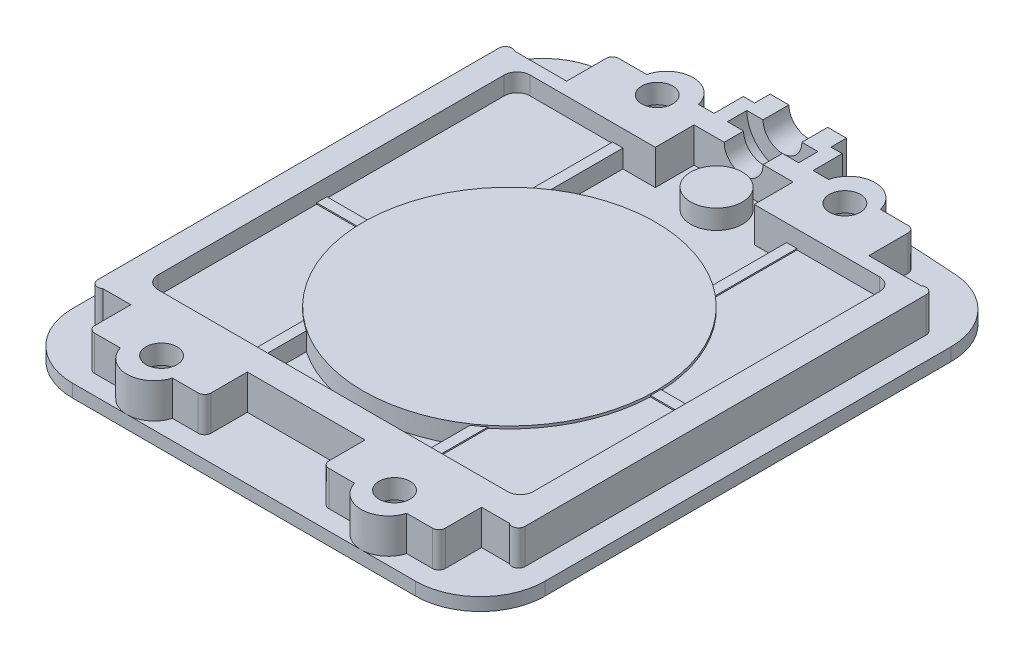
from build123d import *

# Parameters (mm, degrees)
BOSS_EXTRUDE1_DEPTH      = 1
BOSS_EXTRUDE3_DEPTH      = 2.7
BOSS_EXTRUDE3_DEPTH_BACK = 1
BOSS_EXTRUDE4_DEPTH      = 1.3
BOSS_EXTRUDE5_DEPTH      = 0.1
SKETCH_6_R               = 11.3
BOSS_EXTRUDE6_DEPTH      = 1.5
SKETCH_8_R               = 1.2
CUT_EXTRUDE1_DEPTH       = 3.7
SKETCH_9_R               = 1.85
SKETCH_9_R_2             = 9.175
CUT_EXTRUDE2_DEPTH       = 2.2
SKETCH_10_R              = 2
BOSS_EXTRUDE11_DEPTH     = 1.5


with BuildPart() as part:
    # Sketch 1 → Boss-Extrude1 (new body)
    with BuildSketch(Plane(origin=(0, 0, 0), x_dir=(1, 0, 0), z_dir=(0, 1, 0))):
        with BuildLine():
            Line((-13.25, -20.5), (13.25, -20.5))
            ThreePointArc((13.25, -20.5), (16.785533906, -19.035533906), (18.25, -15.5))
            Line((18.25, -15.5), (18.25, 15.890687558))
            ThreePointArc((18.25, 15.890687558), (16.905897578, 19.301613077), (13.59623484, 20.878685296))
            ThreePointArc((13.59623484, 20.878685296), (0, 21.35), (-13.59623484, 20.878685296))
            ThreePointArc((-13.59623484, 20.878685296), (-16.905897578, 19.301613077), (-18.25, 15.890687558))
            Line((-18.25, 15.890687558), (-18.25, -15.5))
            ThreePointArc((-18.25, -15.5), (-16.785533906, -19.035533906), (-13.25, -20.5))
        make_face()
    extrude(amount=BOSS_EXTRUDE1_DEPTH)

    # Sketch 2 → Boss-Extrude3 (add, two sides: drawn at the far end of the back side and taken through both)
    with BuildSketch(Plane(origin=(0, 1, 0), x_dir=(1, 0, 0), z_dir=(0, 1, 0)).offset(-BOSS_EXTRUDE3_DEPTH_BACK)):
        with BuildLine():
            Line((-13.55, -15.702154728), (-15.705804316, -15.702154728))
            ThreePointArc((-15.705804316, -15.702154728), (-16.229411113, -15.749368323), (-16.505804316, -15.302154728))
            Line((-16.505804316, -15.302154728), (-16.505804316, 15.697845272))
            ThreePointArc((-16.505804316, 15.697845272), (-16.229411113, 16.145058868), (-15.705804316, 16.097845272))
            Line((-15.705804316, 16.097845272), (-11.675, 16.097845272))
            Line((-11.675, 16.097845272), (-11.675, 19.137801572))
            ThreePointArc((-11.675, 19.137801572), (-11.528553391, 19.491354963), (-11.175, 19.637801572))
            Line((-11.175, 19.637801572), (-9.025, 19.637801572))
            ThreePointArc((-9.025, 19.637801572), (-7.025, 21.222955871), (-5.025, 19.637801572))
            Line((-5.025, 19.637801572), (-3.825, 19.637801572))
            Line((-3.825, 19.637801572), (-3.825, 21.897845272))
            Line((-3.825, 21.897845272), (-2.95, 21.897845272))
            Line((-2.95, 21.897845272), (-2.95, 23.097845272))
            Line((-2.95, 23.097845272), (2.95, 23.097845272))
            Line((2.95, 23.097845272), (2.95, 21.897845272))
            Line((2.95, 21.897845272), (3.825, 21.897845272))
            Line((3.825, 21.897845272), (3.825, 19.637801572))
            Line((3.825, 19.637801572), (5.025, 19.637801572))
            ThreePointArc((5.025, 19.637801572), (7.025, 21.222955871), (9.025, 19.637801572))
            Line((9.025, 19.637801572), (11.175, 19.637801572))
            ThreePointArc((11.175, 19.637801572), (11.528553391, 19.491354963), (11.675, 19.137801572))
            Line((11.675, 19.137801572), (11.675, 16.097845272))
            Line((11.675, 16.097845272), (15.705804316, 16.097845272))
            ThreePointArc((15.705804316, 16.097845272), (16.229411113, 16.145058868), (16.505804316, 15.697845272))
            Line((16.505804316, 15.697845272), (16.505804316, -15.302154728))
            ThreePointArc((16.505804316, -15.302154728), (16.229411113, -15.749368323), (15.705804316, -15.702154728))
            Line((15.705804316, -15.702154728), (13.55, -15.702154728))
            Line((13.55, -15.702154728), (13.55, -18.5))
            ThreePointArc((13.55, -18.5), (13.403553391, -18.853553391), (13.05, -19))
            Line((13.05, -19), (11.06246118, -19))
            ThreePointArc((11.06246118, -19), (9.05, -20.5), (7.03753882, -19))
            Line((7.03753882, -19), (5.05, -19))
            ThreePointArc((5.05, -19), (4.696446609, -18.853553391), (4.55, -18.5))
            Line((4.55, -18.5), (4.55, -15.702154728))
            Line((4.55, -15.702154728), (-4.55, -15.702154728))
            Line((-4.55, -15.702154728), (-4.55, -18.5))
            ThreePointArc((-4.55, -18.5), (-4.696446609, -18.853553391), (-5.05, -19))
            Line((-5.05, -19), (-7.03753882, -19))
            ThreePointArc((-7.03753882, -19), (-9.05, -20.5), (-11.06246118, -19))
            Line((-11.06246118, -19), (-13.05, -19))
            ThreePointArc((-13.05, -19), (-13.403553391, -18.853553391), (-13.55, -18.5))
            Line((-13.55, -18.5), (-13.55, -15.702154728))
        make_face()
        with BuildLine():
            Line((-14.5, -12.65), (-14.5, 14.097845272))
            ThreePointArc((-14.5, 14.097845272), (-14.207106781, 14.804952053), (-13.5, 15.097845272))
            Line((-13.5, 15.097845272), (-3.825, 15.097845272))
            Line((-3.825, 15.097845272), (-3.825, 18.097845272))
            Line((-3.825, 18.097845272), (3.825, 18.097845272))
            Line((3.825, 18.097845272), (3.825, 15.097845272))
            Line((3.825, 15.097845272), (13.5, 15.097845272))
            ThreePointArc((13.5, 15.097845272), (14.207106781, 14.804952053), (14.5, 14.097845272))
            Line((14.5, 14.097845272), (14.5, -12.65))
            ThreePointArc((14.5, -12.65), (14.207106781, -13.357106781), (13.5, -13.65))
            Line((13.5, -13.65), (-13.5, -13.65))
            ThreePointArc((-13.5, -13.65), (-14.207106781, -13.357106781), (-14.5, -12.65))
        make_face(mode=Mode.SUBTRACT)
    extrude(amount=BOSS_EXTRUDE3_DEPTH + BOSS_EXTRUDE3_DEPTH_BACK)

    # Sketch 4 → Boss-Extrude4 (add)
    with BuildSketch(Plane(origin=(0, 1, 0), x_dir=(1, 0, 0), z_dir=(0, 1, 0))):
        with BuildLine():
            Line((-6.325, 15.097845272), (-6.325, -13.65))
            Line((-6.325, -13.65), (-13.5, -13.65))
            ThreePointArc((-13.5, -13.65), (-14.207106781, -13.357106781), (-14.5, -12.65))
            Line((-14.5, -12.65), (-14.5, 14.097845272))
            ThreePointArc((-14.5, 14.097845272), (-14.207106781, 14.804952053), (-13.5, 15.097845272))
            Line((-13.5, 15.097845272), (-6.325, 15.097845272))
        make_face()
        with BuildLine():
            Line((13.5, -13.65), (6.325, -13.65))
            Line((6.325, -13.65), (6.325, 15.097845272))
            Line((6.325, 15.097845272), (13.5, 15.097845272))
            ThreePointArc((13.5, 15.097845272), (14.207106781, 14.804952053), (14.5, 14.097845272))
            Line((14.5, 14.097845272), (14.5, -12.65))
            ThreePointArc((14.5, -12.65), (14.207106781, -13.357106781), (13.5, -13.65))
        make_face()
    extrude(amount=BOSS_EXTRUDE4_DEPTH)

    # Sketch 5 → Boss-Extrude5 (add)
    with BuildSketch(Plane(origin=(0, 2.3, 0), x_dir=(1, 0, 0), z_dir=(0, 1, 0))):
        Polygon((-6.325, 15.097845272), (-6.325, -13.65), (-7.125, -13.65), (-7.125, -0.4), (-14.5, -0.4), (-14.5, 0.4), (-7.125, 0.4), (-7.125, 15.097845272), align=None)
        Polygon((7.125, -0.4), (7.125, -13.65), (6.325, -13.65), (6.325, 15.097845272), (7.125, 15.097845272), (7.125, 0.4), (14.5, 0.4), (14.5, -0.4), align=None)
    extrude(amount=BOSS_EXTRUDE5_DEPTH)

    # Sketch 6 → Boss-Extrude6 (add)
    with BuildSketch(Plane(origin=(0, 1, 0), x_dir=(1, 0, 0), z_dir=(0, 1, 0))):
        with Locations(Location((0, 0, 0), (0, 0, 55.962560444))):
            Circle(SKETCH_6_R)
    extrude(amount=BOSS_EXTRUDE6_DEPTH)

    # Sketch 7 → Cut-Revolve1 (revolve, cut)
    with BuildSketch(Plane(origin=(0, 0, 0), x_dir=(0, 0, -1), z_dir=(1, 0, 0))):
        Polygon((23.097845272, 3.7), (23.097845272, 2.2), (21.097845272, 2.2), (21.097845272, 0.95), (19.597845272, 0.95), (19.597845272, 2.2), (18.097845272, 2.2), (18.097845272, 3.7), align=None)
    revolve(axis=Axis((0, 3.7, -14.738823172), (0, 0, -1)), mode=Mode.SUBTRACT)

    # Sketch 8 → Cut-Extrude1 (cut)
    with BuildSketch(Plane(origin=(0, 3.7, 0), x_dir=(1, 0, 0), z_dir=(0, 1, 0))):
        with Locations(Location((-7.25, 18.672955871, 0), (0, 0, 270))):
            Circle(SKETCH_8_R)
        with Locations(Location((9.05, -17.927044129, 0), (0, 0, 270))):
            Circle(SKETCH_8_R)
        with Locations(Location((-8.953692371, -17.927044129, 0), (0, 0, 270))):
            Circle(SKETCH_8_R)
        with Locations(Location((7.25, 18.672955871, 0), (0, 0, 270))):
            Circle(SKETCH_8_R)
    extrude(amount=-CUT_EXTRUDE1_DEPTH, mode=Mode.SUBTRACT)

    # Sketch 9 → Cut-Extrude2 (cut)
    with BuildSketch(Plane.XZ):
        with Locations(Location((-8.953692371, 17.927044129, 0), (0, 0, 270))):
            Circle(SKETCH_9_R)
        with Locations(Location((9.05, 17.927044129, 0), (0, 0, 270))):
            Circle(SKETCH_9_R)
        with Locations(Location((-7.25, -18.672955871, 0), (0, 0, 270))):
            Circle(SKETCH_9_R)
        with Locations(Location((7.25, -18.672955871, 0), (0, 0, 270))):
            Circle(SKETCH_9_R)
        with Locations(Location((0, 0, 0), (0, 0, 270))):
            Circle(SKETCH_9_R_2)
    extrude(amount=-CUT_EXTRUDE2_DEPTH, mode=Mode.SUBTRACT)

    # Sketch 10 → Boss-Extrude11 (add)
    with BuildSketch(Plane(origin=(0, 1, 0), x_dir=(1, 0, 0), z_dir=(0, 1, 0))):
        with Locations(Location((0, 16.008968339, 0), (0, 0, 270))):
            Circle(SKETCH_10_R)
    extrude(amount=BOSS_EXTRUDE11_DEPTH)


solid = part.part
